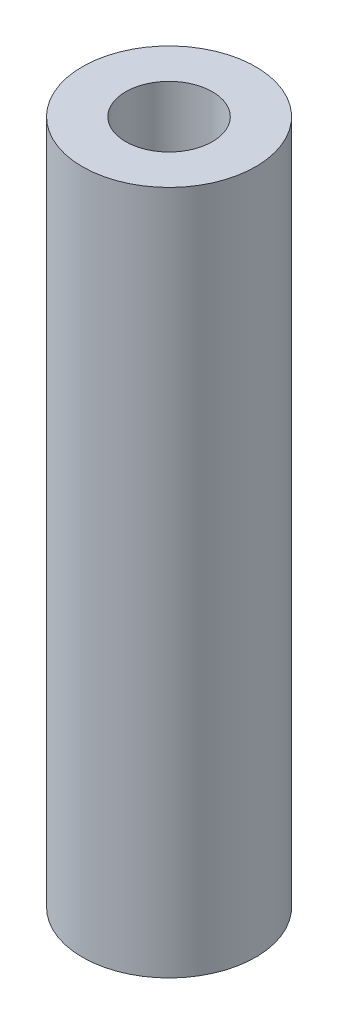
from build123d import *

# Parameters (mm, degrees)
SKETCH1_R           = 10
SKETCH1_R_2         = 5
BOSS_EXTRUDE1_DEPTH = 79


with BuildPart() as part:
    # Sketch1 → Boss-Extrude1 (new body)
    with BuildSketch(Plane(origin=(0, 0, 0), x_dir=(1, 0, 0), z_dir=(0, 1, 0))):
        with Locations(Location((0, 0, 0), (0, 0, 270))):
            Circle(SKETCH1_R)
        with Locations(Location((0, 0, 0), (0, 0, 270))):
            Circle(SKETCH1_R_2, mode=Mode.SUBTRACT)
    extrude(amount=BOSS_EXTRUDE1_DEPTH)


solid = part.part
